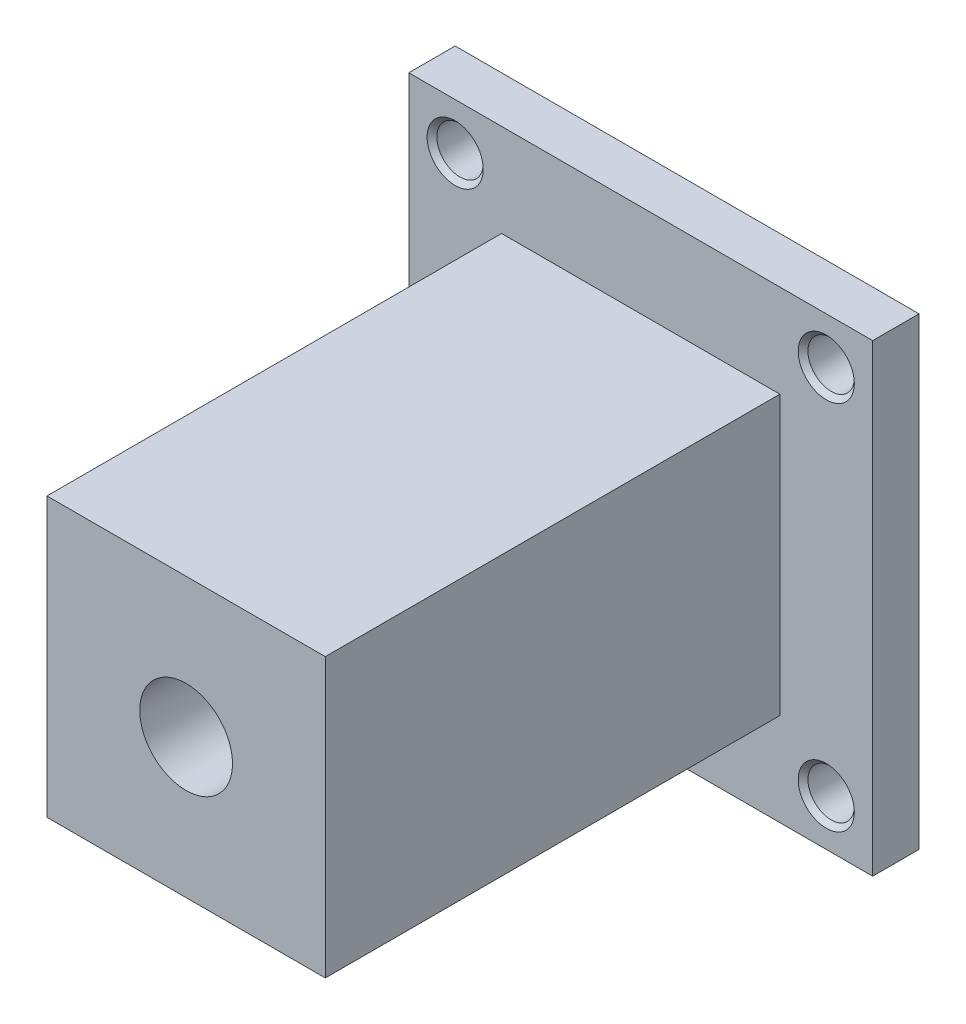
from build123d import *

# Parameters (mm, degrees)
SKETCH_1_W                   = 30
SKETCH_1_H                   = 30
EXTRUDE_1_DEPTH              = 54
SKETCH_2_W                   = 50
SKETCH_2_H                   = 50
EXTRUDE_2_DEPTH              = 5
HOLE_WIZARD_M6_1_D           = 5
HOLE_WIZARD_M6_1_DEPTH       = 13.497848452
HOLE_WIZARD_M6_1_CSINK_D     = 6.05
HOLE_WIZARD_M6_1_CSINK_ANGLE = 90
HOLE_WIZARD_M6_1_TIP         = 1.502151548
SKETCH_6_R                   = 5
CUT_EXTRUDE_1_DEPTH          = 39


with BuildPart() as part:
    # 草图1 → 凸台-拉伸1 (new body)
    with BuildSketch(Plane.XY):
        with Locations((-50, 0)):
            Rectangle(SKETCH_1_W, SKETCH_1_H)
    extrude(amount=EXTRUDE_1_DEPTH)

    # 草图2 → 凸台-拉伸2 (add)
    with BuildSketch(Plane.XY):
        with Locations((-50, 0)):
            Rectangle(SKETCH_2_W, SKETCH_2_H)
    extrude(amount=EXTRUDE_2_DEPTH)

    # M6 螺纹孔1
    with Locations(Plane.XY.offset(5)):
        with Locations((-30, 20), (-70, 20), (-70, -20), (-30, -20)):
            CounterSinkHole(HOLE_WIZARD_M6_1_D / 2, HOLE_WIZARD_M6_1_CSINK_D / 2, depth=HOLE_WIZARD_M6_1_DEPTH, counter_sink_angle=HOLE_WIZARD_M6_1_CSINK_ANGLE)
            with Locations((0, 0, -(HOLE_WIZARD_M6_1_DEPTH + HOLE_WIZARD_M6_1_TIP / 2))):  # 118° drill point
                Cone(0, HOLE_WIZARD_M6_1_D / 2, HOLE_WIZARD_M6_1_TIP, mode=Mode.SUBTRACT)

    # 草图6 → 切除-拉伸1 (cut)
    with BuildSketch(Plane.XY.offset(54)):
        with Locations((-50, 0)):
            Circle(SKETCH_6_R)
    extrude(amount=-CUT_EXTRUDE_1_DEPTH, mode=Mode.SUBTRACT)


solid = part.part
